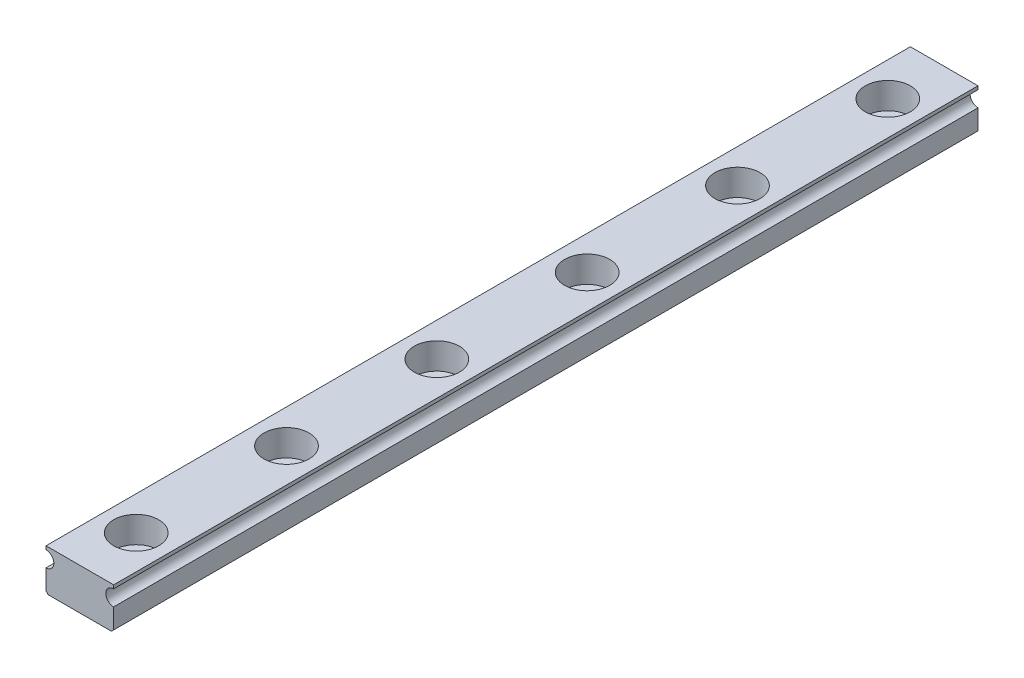
from build123d import *

# Parameters (mm, degrees)
BOSS_EXTRUDE1_DEPTH = 115


with BuildPart() as part:
    # Sketch1 → Boss-Extrude1 (new body)
    with BuildSketch(Plane.XY):
        with BuildLine():
            Line((-4.5, 5.5), (-4.5, 5.04))
            ThreePointArc((-4.5, 5.04), (-3.46, 4), (-4.5, 2.96))
            Line((-4.5, 2.96), (-4.5, 0.296984848))
            Line((-4.5, 0.296984848), (-4.203015152, 0))
            Line((-4.203015152, 0), (4.203015152, 0))
            Line((4.203015152, 0), (4.5, 0.296984848))
            Line((4.5, 0.296984848), (4.5, 2.96))
            ThreePointArc((4.5, 2.96), (3.46, 4), (4.5, 5.04))
            Line((4.5, 5.04), (4.5, 5.5))
            Line((4.5, 5.5), (-4.5, 5.5))
        make_face()
    extrude(amount=BOSS_EXTRUDE1_DEPTH)

    # Sketch2 → Cut-Revolve1 (revolve, cut)
    with BuildSketch(Plane(origin=(0, 0, 0), x_dir=(0, 0, -1), z_dir=(1, 0, 0)), mode=Mode.PRIVATE) as cut_revolve1_sk:
        Polygon((-7.5, 5.5), (-4.5, 5.5), (-4.5, 2), (-5.75, 2), (-5.75, 0), (-7.5, 0), align=None)
    revolve(cut_revolve1_sk.sketch.rotate(Axis((0, 0, 7.5), (0, 1, 0)), 180), axis=Axis((0, 0, 7.5), (0, 1, 0)), mode=Mode.SUBTRACT)

    # Sketch3 → Cut-Revolve2 (revolve, cut)
    with BuildSketch(Plane(origin=(0, 0, 0), x_dir=(0, 0, -1), z_dir=(1, 0, 0)), mode=Mode.PRIVATE) as cut_revolve2_sk:
        Polygon((-107.5, 5.5), (-104.5, 5.5), (-104.5, 2), (-105.75, 2), (-105.75, 0), (-107.5, 0), align=None)
    revolve(cut_revolve2_sk.sketch.rotate(Axis((0, 0, 107.5), (0, 1, 0)), 180), axis=Axis((0, 0, 107.5), (0, 1, 0)), mode=Mode.SUBTRACT)

    # Sketch4 → Cut-Revolve3 (revolve, cut)
    with BuildSketch(Plane(origin=(0, 0, 0), x_dir=(0, 0, -1), z_dir=(1, 0, 0)), mode=Mode.PRIVATE) as cut_revolve3_sk:
        Polygon((-87.5, 5.5), (-84.5, 5.5), (-84.5, 2), (-85.75, 2), (-85.75, 0), (-87.5, 0), align=None)
    revolve(cut_revolve3_sk.sketch.rotate(Axis((0, 0, 87.5), (0, 1, 0)), 180), axis=Axis((0, 0, 87.5), (0, 1, 0)), mode=Mode.SUBTRACT)

    # Sketch5 → Cut-Revolve4 (revolve, cut)
    with BuildSketch(Plane(origin=(0, 0, 0), x_dir=(0, 0, -1), z_dir=(1, 0, 0)), mode=Mode.PRIVATE) as cut_revolve4_sk:
        Polygon((-67.5, 5.5), (-64.5, 5.5), (-64.5, 2), (-65.75, 2), (-65.75, 0), (-67.5, 0), align=None)
    revolve(cut_revolve4_sk.sketch.rotate(Axis((0, 0, 67.5), (0, 1, 0)), 180), axis=Axis((0, 0, 67.5), (0, 1, 0)), mode=Mode.SUBTRACT)

    # Sketch6 → Cut-Revolve5 (revolve, cut)
    with BuildSketch(Plane(origin=(0, 0, 0), x_dir=(0, 0, -1), z_dir=(1, 0, 0)), mode=Mode.PRIVATE) as cut_revolve5_sk:
        Polygon((-47.5, 5.5), (-44.5, 5.5), (-44.5, 2), (-45.75, 2), (-45.75, 0), (-47.5, 0), align=None)
    revolve(cut_revolve5_sk.sketch.rotate(Axis((0, 0, 47.5), (0, 1, 0)), 180), axis=Axis((0, 0, 47.5), (0, 1, 0)), mode=Mode.SUBTRACT)

    # Sketch7 → Cut-Revolve6 (revolve, cut)
    with BuildSketch(Plane(origin=(0, 0, 0), x_dir=(0, 0, -1), z_dir=(1, 0, 0)), mode=Mode.PRIVATE) as cut_revolve6_sk:
        Polygon((-27.5, 5.5), (-24.5, 5.5), (-24.5, 2), (-25.75, 2), (-25.75, 0), (-27.5, 0), align=None)
    revolve(cut_revolve6_sk.sketch.rotate(Axis((0, 0, 27.5), (0, 1, 0)), 180), axis=Axis((0, 0, 27.5), (0, 1, 0)), mode=Mode.SUBTRACT)


solid = part.part
